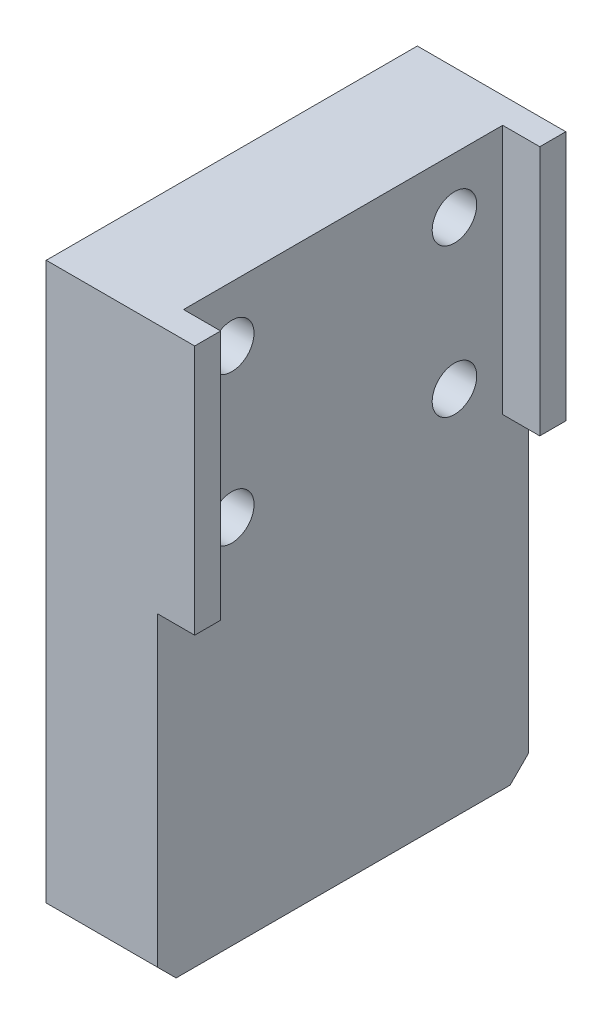
from build123d import *

# Parameters (mm, degrees)
SKETCH2_W                                            = 20
SKETCH2_H                                            = 31
BOSS_EXTRUDE1_DEPTH                                  = 6
SKETCH3_W                                            = 1.4
SKETCH3_H                                            = 31
BOSS_EXTRUDE2_DEPTH                                  = 2
SKETCH4_W                                            = 2
SKETCH4_H                                            = 17.5
CUT_EXTRUDE1_DEPTH                                   = 27.537709019
CBORE_FOR_M2_HEXAGON_SOCKET_HEAD_CAP_SCR_D           = 2.4
CBORE_FOR_M2_HEXAGON_SOCKET_HEAD_CAP_SCR_DEPTH       = 10.1
CBORE_FOR_M2_HEXAGON_SOCKET_HEAD_CAP_SCR_CBORE_D     = 4.3
CBORE_FOR_M2_HEXAGON_SOCKET_HEAD_CAP_SCR_CBORE_DEPTH = 2.3
CBORE_FOR_M2_HEXAGON_SOCKET_HEAD_CAP_SCR_TIP         = 0.721032743
M3_TAPPED_HOLE1_D                                    = 2.5
M3_TAPPED_HOLE1_DEPTH                                = 7.5
M3_TAPPED_HOLE1_TIP                                  = 0.751075774
CHAMFER1_SIZE                                        = 1


with BuildPart() as part:
    # Sketch2 → Boss-Extrude1 (new body)
    with BuildSketch(Plane(origin=(0, 0, 0), x_dir=(0, 0, -1), z_dir=(1, 0, 0))):
        Rectangle(SKETCH2_W, SKETCH2_H)
    extrude(amount=BOSS_EXTRUDE1_DEPTH)

    # Sketch3 → Boss-Extrude2 (add)
    with BuildSketch(Plane(origin=(6, 0, 0), x_dir=(0, 0, -1), z_dir=(1, 0, 0))):
        with Locations((-9.3, 0)):
            Rectangle(SKETCH3_W, SKETCH3_H)
        with Locations((9.3, 0)):
            Rectangle(SKETCH3_W, SKETCH3_H)
    extrude(amount=BOSS_EXTRUDE2_DEPTH)

    # Sketch4 → Cut-Extrude1 (cut, through all)
    with BuildSketch(Plane.XY.offset(10)):
        with Locations((7, -6.75)):
            Rectangle(SKETCH4_W, SKETCH4_H)
    extrude(amount=-CUT_EXTRUDE1_DEPTH, mode=Mode.SUBTRACT)

    # CBORE for M2 Hexagon socket head cap screws1
    with Locations(Plane.ZY):
        with Locations((6, 12.5), (-6, 12.5), (-6, 4.5), (6, 4.5)):
            CounterBoreHole(CBORE_FOR_M2_HEXAGON_SOCKET_HEAD_CAP_SCR_D / 2, CBORE_FOR_M2_HEXAGON_SOCKET_HEAD_CAP_SCR_CBORE_D / 2, CBORE_FOR_M2_HEXAGON_SOCKET_HEAD_CAP_SCR_CBORE_DEPTH, depth=CBORE_FOR_M2_HEXAGON_SOCKET_HEAD_CAP_SCR_DEPTH)
            with Locations((0, 0, -(CBORE_FOR_M2_HEXAGON_SOCKET_HEAD_CAP_SCR_DEPTH + CBORE_FOR_M2_HEXAGON_SOCKET_HEAD_CAP_SCR_TIP / 2))):  # 118° drill point
                Cone(0, CBORE_FOR_M2_HEXAGON_SOCKET_HEAD_CAP_SCR_D / 2, CBORE_FOR_M2_HEXAGON_SOCKET_HEAD_CAP_SCR_TIP, mode=Mode.SUBTRACT)

    # M3 Tapped Hole1
    with Locations(Plane(origin=(0, -15.5, 0), x_dir=(-1, 0, 0), z_dir=(0, -1, 0))):
        with Locations((-3, 5), (-3, -5)):
            Hole(M3_TAPPED_HOLE1_D / 2, depth=M3_TAPPED_HOLE1_DEPTH)
            with Locations((0, 0, -(M3_TAPPED_HOLE1_DEPTH + M3_TAPPED_HOLE1_TIP / 2))):  # 118° drill point
                Cone(0, M3_TAPPED_HOLE1_D / 2, M3_TAPPED_HOLE1_TIP, mode=Mode.SUBTRACT)

    # Chamfer1
    chamfer1_edges = [part.edges().sort_by_distance(p)[0] for p in [
        (3, -15.5, -10),
        (3, -15.5, 10),
    ]]
    chamfer(chamfer1_edges, length=CHAMFER1_SIZE)


solid = part.part
